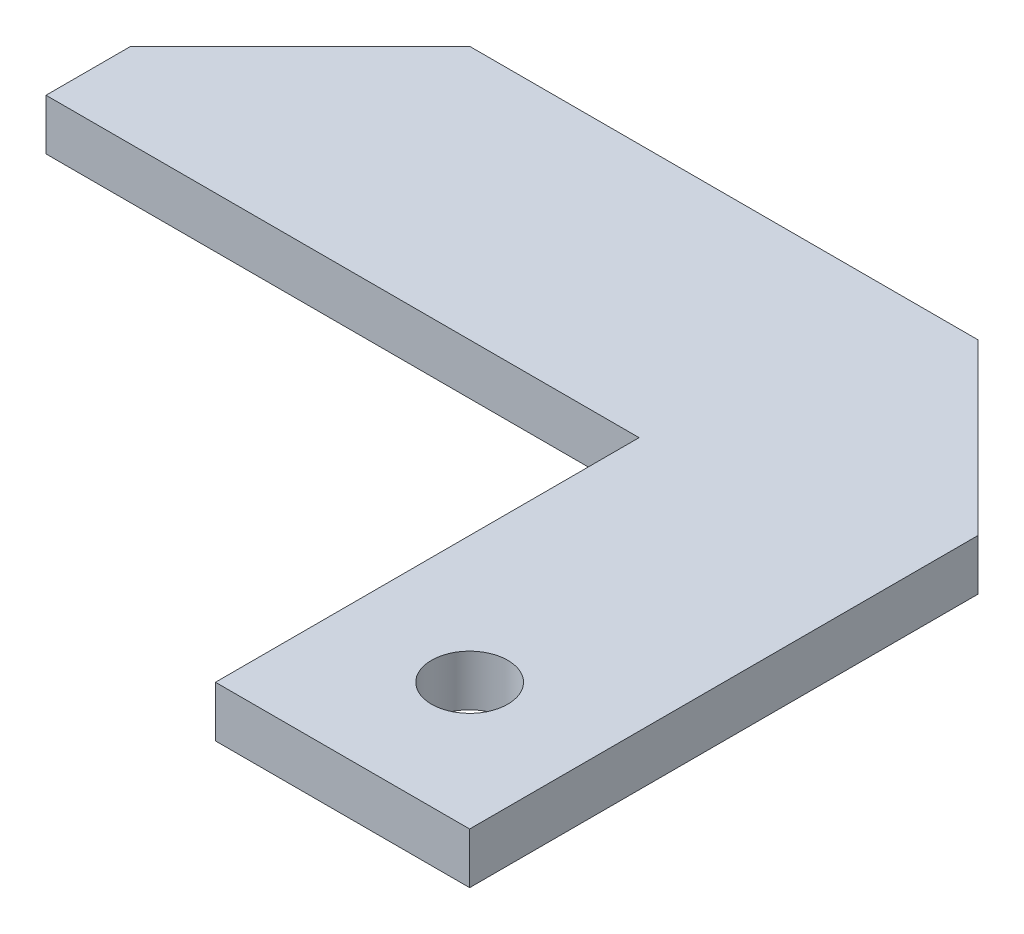
SolidWorks part; units mm, degrees
material "K"
ref_plane "Front" through (0, 0, 0) normal (0, 0, 1) x (1, 0, 0)
ref_plane "Top" through (0, 0, 0) normal (0, 1, 0) x (1, 0, 0)
ref_plane "Right" through (0, 0, 0) normal (1, 0, 0) x (0, 0, -1)
sketch "Sketch1" plane through (0, 0, 0) normal (0, 1, 0) x (1, 0, 0)
  line L0 (-18.0769, 61.9231) -> (81.9231, 61.9231)
  line L1 (81.9231, 61.9231) -> (81.9231, -18.0769)
  line L2 (81.9231, -18.0769) -> (51.9231, -18.0769)
  line L3 (51.9231, -18.0769) -> (51.9231, 31.9231)
  line L4 (51.9231, 31.9231) -> (-18.0769, 31.9231)
  line L5 (-18.0769, 31.9231) -> (-18.0769, 61.9231)
  dimension "D1" = 30
  dimension "D2" = 80
  dimension "D3" = 100
  dimension "D4" = 30
extrude "Boss-Extrude1" add sketch "Sketch1" along normal blind 6
sketch "Sketch2" plane through (0, 6, 0) normal (0, 1, 0) x (1, 0, 0)
  line L0 (66.9231, -18.0769) -> (66.9231, 27.3292) construction
  line L1 (51.9231, -18.0769) -> (81.9231, -18.0769) construction
  circle A0 centre (66.9231, -3.0769) radius 4.5
  dimension "D1" = 9
  dimension "D2" = 15
extrude "Cut-Extrude1" cut sketch "Sketch2" against normal blind 6
chamfer "Chamfer1" distance 20 angle 45 1 edges at (-18.0769, 3, -61.9231)
chamfer "Chamfer2" distance 20 angle 45 1 edges at (81.9231, 3, -61.9231)
equation "\"零件重量\"= IIF ( \"SW-质量\" > 100 , int ( \"SW-质量\" ) , \"SW-质量\" )"
